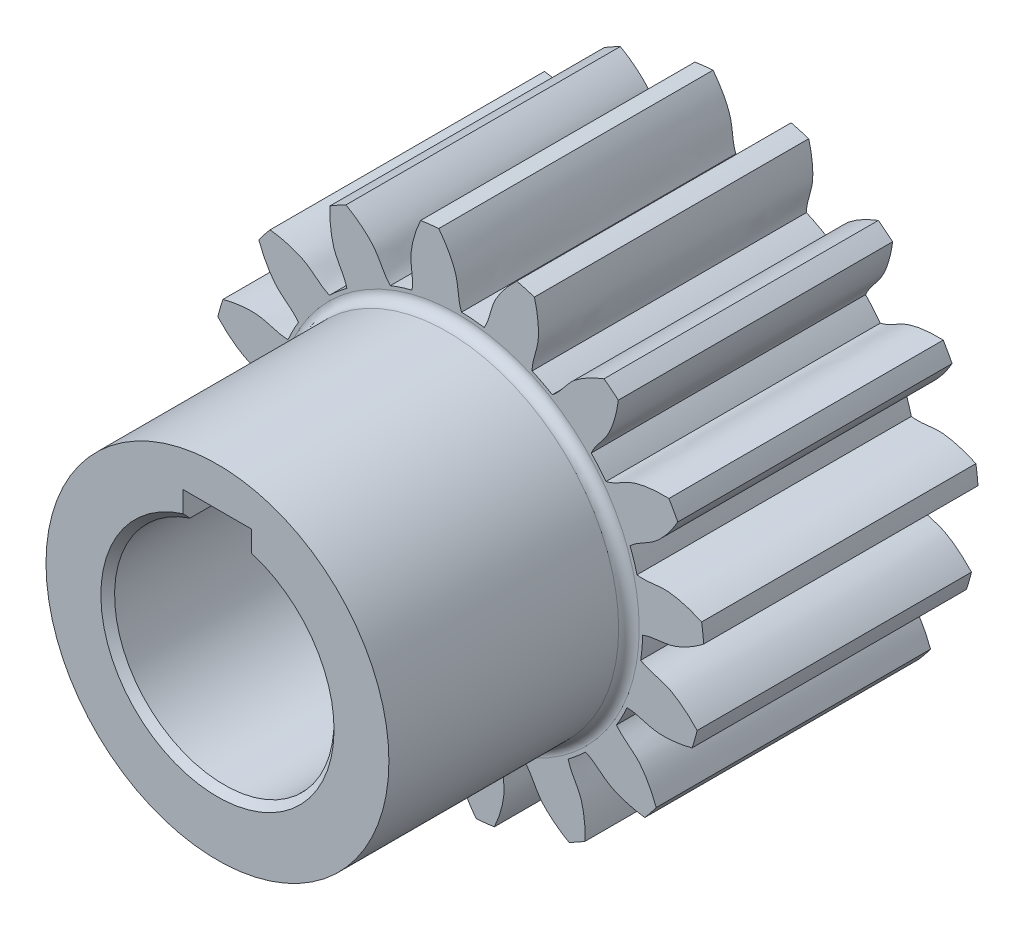
from build123d import *

# Parameters (mm, degrees)
SKETCH1_R           = 27
SKETCH1_R_2         = 16
BOSS_EXTRUDE1_DEPTH = 40
BOSS_EXTRUDE2_DEPTH = 40
CIRPATTERN1_COUNT   = 16
SKETCH3_R           = 25
SKETCH3_R_2         = 16
BOSS_EXTRUDE3_DEPTH = 35
FILLET1_R           = 1.5
SKETCH4_R           = 21
CUT_EXTRUDE1_DEPTH  = 8
CHAMFER1_SIZE       = 1
CUT_EXTRUDE2_REACH  = 92.565
SKETCH5_W           = 10
SKETCH5_H           = 6.6


with BuildPart() as part:
    # Sketch1 → Boss-Extrude1 (new body)
    with BuildSketch(Plane.XY):
        Circle(SKETCH1_R)
        Circle(SKETCH1_R_2, mode=Mode.SUBTRACT)
    extrude(amount=BOSS_EXTRUDE1_DEPTH)

    # Sketch2 → Boss-Extrude2 (add)
    with BuildSketch(Plane.XY):
        with BuildLine():
            ThreePointArc((35.595422314, 5.381998727), (35.77008104, 4.062179512), (35.895820084, 2.736804801))
            add(Edge.make_bspline(
                [(35.895820084, 2.736804801), (35.171538942, 2.178997759), (34.047196938, 1.420458911), (32.45827874, 0.64438799), (30.301464937, -0.185622899), (28.343240331, -0.038024245), (26.993578575, -0.588825693)],
                knots=[0, 0, 0, 0, 0.28472745, 0.419800154, 0.549994158, 1, 1, 1, 1], degree=3))
            ThreePointArc((26.993578575, -0.588825693), (26.82756078, 3.046634634), (26.17415231, 6.626745117))
            add(Edge.make_bspline(
                [(35.595422314, 5.381998727), (34.764504929, 5.763191811), (33.498703058, 6.250297294), (31.776224105, 6.650314002), (29.488215745, 6.975554842), (27.612954107, 6.392611654), (26.17415231, 6.626745117)],
                knots=[0, 0, 0, 0, 0.28472745, 0.419800154, 0.549994158, 1, 1, 1, 1], degree=3))
        make_face()
    boss_extrude2 = extrude(amount=BOSS_EXTRUDE2_DEPTH)

    # CirPattern1: Boss-Extrude2 ×16 about axis
    cirpattern1_axis = Axis((0, 0, 40), (0, 0, -1))
    for i in range(1, CIRPATTERN1_COUNT):
        add(boss_extrude2.rotate(cirpattern1_axis, i * 360 / CIRPATTERN1_COUNT))

    # Sketch3 → Boss-Extrude3 (add)
    with BuildSketch(Plane.XY.offset(40)):
        Circle(SKETCH3_R)
        Circle(SKETCH3_R_2, mode=Mode.SUBTRACT)
    extrude(amount=BOSS_EXTRUDE3_DEPTH)

    # Fillet1
    fillet1_edges = [part.edges().sort_by_distance(p)[0] for p in [
        (-25, 0, 40),
    ]]
    fillet(fillet1_edges, radius=FILLET1_R)

    # Sketch4 → Cut-Extrude1 (cut)
    with BuildSketch(Plane(origin=(0, 0, 0), x_dir=(-1, 0, 0), z_dir=(0, 0, -1))):
        Circle(SKETCH4_R)
    extrude(amount=-CUT_EXTRUDE1_DEPTH, mode=Mode.SUBTRACT)

    # Chamfer1
    chamfer1_edges = [part.edges().sort_by_distance(p)[0] for p in [
        (-16, 0, 75),
        (-16, 0, 8),
        (21, 0, 0),
    ]]
    chamfer(chamfer1_edges, length=CHAMFER1_SIZE)

    # Sketch5 → Cut-Extrude2 (cut, up to next)
    with BuildSketch(Plane.XY.offset(75), mode=Mode.PRIVATE) as cut_extrude2_sk1:
        with Locations((0, 16)):
            Rectangle(SKETCH5_W, SKETCH5_H)
    cut_extrude2_tool1 = extrude(cut_extrude2_sk1.sketch, amount=-CUT_EXTRUDE2_REACH, mode=Mode.PRIVATE) & part.part
    add(cut_extrude2_tool1.solids().sort_by_distance((0, 16, 75))[0], mode=Mode.SUBTRACT)


solid = part.part
